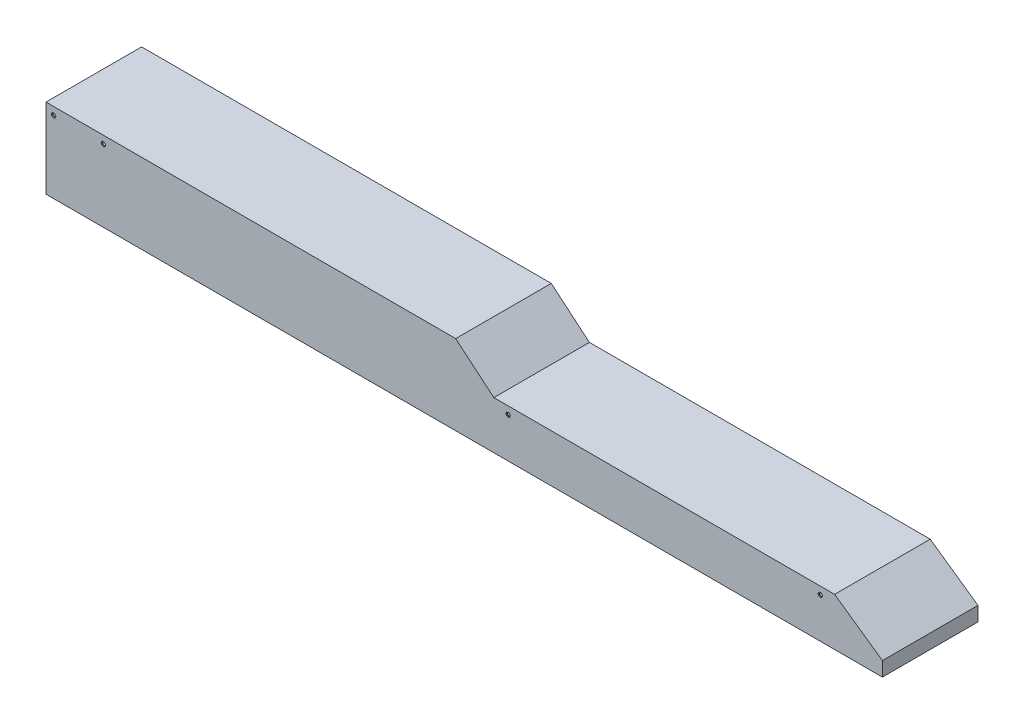
SolidWorks part; units mm, degrees
ref_plane "前视" through (0, 0, 0) normal (0, 0, 1) x (1, 0, 0)
ref_plane "上视" through (0, 0, 0) normal (0, 1, 0) x (1, 0, 0)
ref_plane "右视" through (0, 0, 0) normal (1, 0, 0) x (0, 0, -1)
sketch "草图1" plane through (0, 0, 0) normal (0, 0, 1) x (1, 0, 0)
  line L0 (0, 0) -> (-35.1708, 0) construction
  line L1 (0, 0) -> (0, 39.168) construction
  line L2 (-1750, 0) -> (0, 0)
  line L3 (-1750, 0) -> (-1750, 167)
  line L4 (-1750, 167) -> (-892.8475, 167)
  line L5 (0, 0) -> (0, 30)
  line L8 (-99.9704, 100) -> (0, 30)
  line L9 (-99.9704, 100) -> (-813, 100)
  line L10 (-892.8475, 167) -> (-813, 100)
  dimension "D1" = 1750
  dimension "D2" = 30
  dimension "D3" = 145
  dimension "D4" = 813
  dimension "D5" = 140
  dimension "D6" = 167
  dimension "D7" = 100
extrude "凸台-拉伸1" add sketch "草图1" along normal mid plane 200
shell "抽壳1" thickness 2
sketch "草图2" plane through (0, 0, 0) normal (0, -1, 0) x (1, 0, 0)
  line L10 (-44, 70) -> (-1706, 70)
  line L11 (-1706, 70) -> (-1706, -70)
  line L12 (-1706, -70) -> (-44, -70)
  line L13 (-44, 70) -> (-44, -70)
  line L14 (0, -100) -> (0, 100)
  line L15 (-1750, -100) -> (0, -100)
  line L16 (-1750, 100) -> (-1750, -100)
  line L17 (0, 100) -> (-1750, 100)
  line L18 (0, -100) -> (0, 100)
  line L19 (-1750, -100) -> (0, -100)
  line L20 (-1750, 100) -> (-1750, -100)
  line L21 (0, 100) -> (-1750, 100)
  line L23 (-30, 70) -> (-1720, 70) construction
  line L24 (-1720, -70) -> (-30, -70) construction
  line L26 (-1720, 70) -> (-1720, -70) construction
  line L27 (-30, -70) -> (-30, 70) construction
  dimension "D2" = 30
  dimension "D3" = 44
  dimension "D4" = 44
  dimension "D1" = 0
extrude "凸台-拉伸2" add sketch "草图2" against normal blind 2
sketch "草图3" plane through (0, 0, 0) normal (0, -1, 0) x (1, 0, 0)
  line L0 (-30, 84) -> (-30, -84) construction
  line L1 (0, 100) -> (0, -100) construction
  line L2 (-1720, 0) -> (56.3106, 0) construction
  line L13 (-1750, 100) -> (-1750, -100) construction
  line L19 (-1720, -84) -> (-30, -84) construction
  line L20 (-1720, 84) -> (-1720, -84) construction
  line L21 (-30, 84) -> (-1720, 84) construction
  circle A0 centre (-1720, 84) radius 4.5
  circle A1 centre (-1156.6667, 84) radius 4.5
  circle A2 centre (-593.3333, 84) radius 4.5
  circle A3 centre (-30, 84) radius 4.5
  circle A4 centre (-30, -84) radius 4.5
  circle A5 centre (-593.3333, -84) radius 4.5
  circle A6 centre (-1156.6667, -84) radius 4.5
  circle A7 centre (-1720, -84) radius 4.5
  dimension "D2" = 9
  dimension "D1" = 9
  dimension "D6" = 9
  dimension "D7" = 9
  dimension "D8" = 563.3333
  dimension "D9" = 563.3333
  dimension "D10" = 30
  dimension "D5" = 30
  dimension "D4" = 2
extrude "切除-拉伸1" cut sketch "草图3" against normal blind 2
sketch "草图4" plane through (0, 2, 0) normal (0, 1, 0) x (1, 0, 0)
  line L1 (-1713.923, -87.5086) -> (-1713.923, -80.4914)
  line L2 (-1713.923, -80.4914) -> (-1720, -76.9828)
  line L3 (-1720, -76.9828) -> (-1726.077, -80.4914)
  line L4 (-1726.077, -80.4914) -> (-1726.077, -87.5086)
  line L5 (-1726.077, -87.5086) -> (-1720, -91.0172)
  line L6 (-1720, -91.0172) -> (-1713.923, -87.5086)
  line L7 (-1720, 92.7031) -> (-1727.5371, 88.3516)
  line L8 (-1727.5371, 88.3516) -> (-1727.5371, 79.6484)
  line L9 (-1727.5371, 79.6484) -> (-1720, 75.2969)
  line L10 (-1720, 75.2969) -> (-1712.4629, 79.6484)
  line L11 (-1712.4629, 79.6484) -> (-1712.4629, 88.3516)
  line L12 (-1712.4629, 88.3516) -> (-1720, 92.7031)
  line L13 (-1156.6667, 92.7031) -> (-1164.2038, 88.3516)
  line L14 (-1164.2038, 88.3516) -> (-1164.2038, 79.6484)
  line L15 (-1164.2038, 79.6484) -> (-1156.6667, 75.2969)
  line L16 (-1156.6667, 75.2969) -> (-1149.1295, 79.6484)
  line L17 (-1149.1295, 79.6484) -> (-1149.1295, 88.3516)
  line L18 (-1149.1295, 88.3516) -> (-1156.6667, 92.7031)
  line L19 (-1156.6667, -76.9828) -> (-1162.7437, -80.4914)
  line L20 (-1162.7437, -80.4914) -> (-1162.7437, -87.5086)
  line L21 (-1162.7437, -87.5086) -> (-1156.6667, -91.0172)
  line L22 (-1156.6667, -91.0172) -> (-1150.5896, -87.5086)
  line L23 (-1150.5896, -87.5086) -> (-1150.5896, -80.4914)
  line L24 (-1150.5896, -80.4914) -> (-1156.6667, -76.9828)
  line L25 (-593.3333, -76.9828) -> (-599.4104, -80.4914)
  line L26 (-599.4104, -80.4914) -> (-599.4104, -87.5086)
  line L27 (-599.4104, -87.5086) -> (-593.3333, -91.0172)
  line L28 (-593.3333, -91.0172) -> (-587.2563, -87.5086)
  line L29 (-587.2563, -87.5086) -> (-587.2563, -80.4914)
  line L30 (-587.2563, -80.4914) -> (-593.3333, -76.9828)
  line L31 (-30, -76.9828) -> (-36.077, -80.4914)
  line L32 (-36.077, -80.4914) -> (-36.077, -87.5086)
  line L33 (-36.077, -87.5086) -> (-30, -91.0172)
  line L34 (-30, -91.0172) -> (-23.923, -87.5086)
  line L35 (-23.923, -87.5086) -> (-23.923, -80.4914)
  line L36 (-23.923, -80.4914) -> (-30, -76.9828)
  line L37 (-30, 92.7031) -> (-37.5371, 88.3516)
  line L38 (-37.5371, 88.3516) -> (-37.5371, 79.6484)
  line L39 (-37.5371, 79.6484) -> (-30, 75.2969)
  line L40 (-30, 75.2969) -> (-22.4629, 79.6484)
  line L41 (-22.4629, 79.6484) -> (-22.4629, 88.3516)
  line L42 (-22.4629, 88.3516) -> (-30, 92.7031)
  line L43 (-593.3333, 92.7031) -> (-600.8705, 88.3516)
  line L44 (-600.8705, 88.3516) -> (-600.8705, 79.6484)
  line L45 (-600.8705, 79.6484) -> (-593.3333, 75.2969)
  line L46 (-593.3333, 75.2969) -> (-585.7962, 79.6484)
  line L47 (-585.7962, 79.6484) -> (-585.7962, 88.3516)
  line L48 (-585.7962, 88.3516) -> (-593.3333, 92.7031)
  circle A0 centre (-1720, -84) radius 6.077 construction
  circle A1 centre (-1720, 84) radius 7.5371 construction
  circle A2 centre (-1156.6667, 84) radius 7.5371 construction
  circle A3 centre (-1156.6667, -84) radius 6.077 construction
  circle A4 centre (-593.3333, -84) radius 6.077 construction
  circle A5 centre (-30, -84) radius 6.077 construction
  circle A6 centre (-30, 84) radius 7.5371 construction
  circle A7 centre (-593.3333, 84) radius 7.5371 construction
  dimension "D2" = 2
extrude "凸台-拉伸4" add sketch "草图4" along normal blind 8
hole_wizard "M8 螺纹孔1" positions "草图6" profile "草图5" tap size "M8" standard "GB"
sketch "草图6" plane through (0, 0, 0) normal (0, -1, 0) x (1, 0, 0)
  point P0 (-1720, 84)
  point P1 (-1720, -84)
  point P3 (-1156.6667, -84)
  point P5 (-1156.6667, 84)
  point P7 (-593.3333, 84)
  point P9 (-593.3333, -84)
  point P11 (-30, 84)
  point P13 (-30, -84)
sketch "草图5" plane through (-1720, 0, 84) normal (1, 0, 0) x (0, 0, -1)
  line L0 (0, 0) -> (0, 21.7929)
  line L1 (0, 21.7929) -> (3.4, 19.75)
  line L2 (3.4, 19.75) -> (3.4, 0)
  line L5 (3.4, 0) -> (0, 0)
  line L10 (0, 21.7929) -> (-3.4, 19.75) construction
  line L11 (0, -6.35) -> (0, 107.95) construction
  dimension "螺纹孔钻头直径" = 6.8
  dimension "螺纹孔钻头深度" = 19.75
  dimension "导头角度" = 118
cosmetic thread "孔螺蚊线19" parameters "D1"=10, "D2"=8
cosmetic thread "孔螺蚊线22" parameters "D1"=10, "D2"=8
cosmetic thread "孔螺蚊线23" parameters "D1"=10, "D2"=8
cosmetic thread "孔螺蚊线24" parameters "D1"=10, "D2"=8
cosmetic thread "孔螺蚊线25" parameters "D1"=10, "D2"=8
cosmetic thread "孔螺蚊线26" parameters "D1"=10, "D2"=8
cosmetic thread "孔螺蚊线27" parameters "D1"=10, "D2"=8
cosmetic thread "孔螺蚊线28" parameters "D1"=10, "D2"=8
sketch "草图8" plane through (0, 0, 100) normal (0, 0, 1) x (1, 0, 0)
  line L4 (-813, 100) -> (-813, -70.66) construction
  line L5 (-1734, 151) -> (-1734, 0)
  line L6 (-892.8475, 151) -> (-1734, 151)
  line L7 (-1734, 151) -> (-1734, 0) construction
  line L8 (-892.8475, 151) -> (-1734, 151) construction
  line L9 (-99.9704, 84) -> (-813, 84)
  line L10 (-99.9704, 84) -> (-813, 84) construction
  line L11 (-99.9704, 100) -> (-99.9704, -59.0324) construction
  line L12 (-783, 100) -> (-783, -70.66) construction
  line L13 (-129.9704, 100) -> (-129.9704, -59.0324) construction
  circle A0 centre (-1734, 151) radius 4.5
  circle A1 centre (-1630, 151) radius 4.5
  circle A2 centre (-783, 84) radius 4.5
  circle A3 centre (-129.9704, 84) radius 4.5
  dimension "D2" = 9
  dimension "D3" = 9
  dimension "D4" = 104
  dimension "D8" = 9
  dimension "D9" = 9
  dimension "D1" = 16
  dimension "D5" = 16
  dimension "D6" = 30
  dimension "D7" = 30
extrude "切除-拉伸2" cut sketch "草图8" against normal blind 8
sketch "草图9" plane through (0, 0, 98) normal (0, 0, -1) x (-1, 0, 0)
  line L1 (1630, 161.199) -> (1621.1674, 156.0995)
  line L2 (1621.1674, 156.0995) -> (1621.1674, 145.9005)
  line L3 (1621.1674, 145.9005) -> (1630, 140.801)
  line L4 (1630, 140.801) -> (1638.8326, 145.9005)
  line L5 (1638.8326, 145.9005) -> (1638.8326, 156.0995)
  line L6 (1638.8326, 156.0995) -> (1630, 161.199)
  line L7 (1734, 159.8981) -> (1726.294, 155.4491)
  line L8 (1726.294, 155.4491) -> (1726.294, 146.5509)
  line L9 (1726.294, 146.5509) -> (1734, 142.1019)
  line L10 (1734, 142.1019) -> (1741.706, 146.5509)
  line L11 (1741.706, 146.5509) -> (1741.706, 155.4491)
  line L12 (1741.706, 155.4491) -> (1734, 159.8981)
  line L13 (783, 90.8947) -> (777.029, 87.4474)
  line L14 (777.029, 87.4474) -> (777.029, 80.5526)
  line L15 (777.029, 80.5526) -> (783, 77.1053)
  line L16 (783, 77.1053) -> (788.971, 80.5526)
  line L17 (788.971, 80.5526) -> (788.971, 87.4474)
  line L18 (788.971, 87.4474) -> (783, 90.8947)
  line L19 (129.9704, 92.6744) -> (122.4581, 88.3372)
  line L20 (122.4581, 88.3372) -> (122.4581, 79.6628)
  line L21 (122.4581, 79.6628) -> (129.9704, 75.3256)
  line L22 (129.9704, 75.3256) -> (137.4826, 79.6628)
  line L23 (137.4826, 79.6628) -> (137.4826, 88.3372)
  line L24 (137.4826, 88.3372) -> (129.9704, 92.6744)
  circle A0 centre (1630, 151) radius 8.8326 construction
  circle A1 centre (1734, 151) radius 7.706 construction
  circle A2 centre (783, 84) radius 5.971 construction
  circle A3 centre (129.9704, 84) radius 7.5123 construction
extrude "凸台-拉伸5" add sketch "草图9" along normal blind 8
hole_wizard "M8 螺纹孔2" positions "草图11" profile "草图10" tap size "M8" standard "GB"
sketch "草图11" plane through (0, 0, 100) normal (0, 0, 1) x (1, 0, 0)
  point P0 (-1630, 151)
  point P1 (-1734, 151)
  point P8 (-783, 84)
  point P10 (-129.9704, 84)
sketch "草图10" plane through (-1630, 151, 100) normal (1, 0, 0) x (0, -1, 0)
  line L0 (0, 0) -> (0, 21.7929)
  line L1 (0, 21.7929) -> (3.4, 19.75)
  line L2 (3.4, 19.75) -> (3.4, 0)
  line L5 (3.4, 0) -> (0, 0)
  line L10 (0, 21.7929) -> (-3.4, 19.75) construction
  line L11 (0, -6.35) -> (0, 107.95) construction
  dimension "螺纹孔钻头直径" = 6.8
  dimension "螺纹孔钻头深度" = 19.75
  dimension "导头角度" = 118
cosmetic thread "孔螺蚊线15" parameters "D1"=10, "D2"=8
cosmetic thread "孔螺蚊线16" parameters "D1"=10, "D2"=8
cosmetic thread "孔螺蚊线20" parameters "D1"=10, "D2"=8
cosmetic thread "孔螺蚊线21" parameters "D1"=10, "D2"=8
